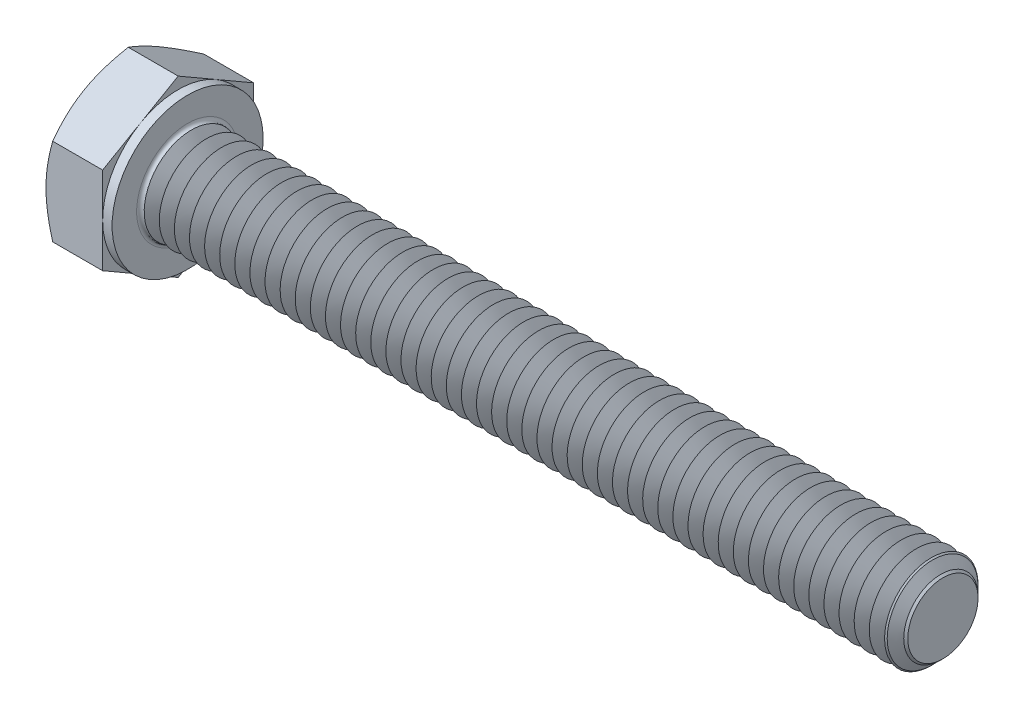
SolidWorks part; units mm, degrees
extrude "Boss-Extrude" add sketch "Sketch1" along normal blind 3.5
sketch "Sketch1" plane through (0, 0, 0) normal (1, 0, 0) x (0, 0, -1)
  line L0 (4, 2.3094) -> (4, -2.3094)
  line L1 (-4, 2.3094) -> (-4, -2.3094)
  line L2 (4, -2.3094) -> (0, -4.6188)
  line L3 (0, -4.6188) -> (-4, -2.3094)
  line L4 (4, 2.3094) -> (0, 4.6188)
  line L5 (0, 4.6188) -> (-4, 2.3094)
revolve "Cut-Revolve1" cut sketch "Sketch3" angle 360 about L6
sketch "Sketch3" plane through (0, 0, 0) normal (0, 0, 1) x (1, 0, 0)
  line L0 (0, 4) -> (3.244, 9.6188)
  line L1 (0, 4.6188) -> (0, 2.3094) construction
  line L2 (3.244, 9.6188) -> (3.244, 14.6188)
  line L3 (3.244, 14.6188) -> (-10, 14.6188)
  line L4 (-10, 14.6188) -> (-10, 4)
  line L5 (-10, 4) -> (0, 4)
  line L6 (0, 0) -> (99.06, 0) construction
  line L7 (3.5, 4.6188) -> (0, 4.6188) construction
revolve "Boss-Revolve1" add sketch "Sketch2" angle 360 about L7
sketch "Sketch2" plane through (0, 0, 0) normal (0, 0, 1) x (1, 0, 0)
  line L0 (0, 2.3094) -> (0, -2.3094) construction
  line L1 (0, 0) -> (43.5, 0)
  line L2 (0, 0) -> (0, 2.5)
  line L3 (0, 2.5) -> (43.5, 2.5)
  line L4 (43.5, 0) -> (43.5, 1.8072)
  line L5 (3.5, 4.6188) -> (3.5, 2.3094) construction
  line L7 (0, 0) -> (96.52, 0) construction
  line L8 (43.5, -1.8072) -> (90.335, -2.5) construction
  line L9 (0, -2.5) -> (90.335, -2.5) construction
  line L10 (4.3, 15.24) -> (4.3, -1.27) construction
  line L11 (3.5, 15.24) -> (3.5, -1.27) construction
  line L12 (3.5, 2.3094) -> (3.5, -2.3094) construction
  line L14 (43.5, 2.5) -> (43.5, 1.8072)
  dimension "l" = 40
  dimension "m" = 5
  dimension "Minor_dia" = 3.6144
  dimension "p" = 0.8
  dimension "h" = 40
cosmetic thread "Helix1" parameters "Thread_length"=39.2, "Thread_minor"=3.6144
ref_plane "Front Plane" through (0, 0, 0) normal (0, 0, 1) x (1, 0, 0)
ref_plane "Top Plane" through (0, 0, 0) normal (0, 1, 0) x (1, 0, 0)
ref_plane "Right Plane" through (0, 0, 0) normal (1, 0, 0) x (0, 0, -1)
sketch "Sketch5" plane through (0, 0, 0) normal (0, 0, 1) x (1, 0, 0)
  line L0 (3.5, 4) -> (0.256, 9.6188)
  line L1 (3.5, 4.6188) -> (3.5, 2.3094) construction
  line L2 (0.256, 9.6188) -> (0.256, 14.6188)
  line L3 (0.256, 14.6188) -> (10.256, 14.6188)
  line L4 (10.256, 14.6188) -> (10.256, 4)
  line L5 (10.256, 4) -> (3.5, 4)
  line L7 (3.5, 4.6188) -> (0.3573, 4.6188) construction
  line L8 (0, 0) -> (99.06, 0) construction
  line L9 (0, 0) -> (99.06, 0) construction
revolve "Cut-Revolve2" cut sketch "Sketch5" angle 360 about L8
sketch "Sketch4" plane through (0, 0, 0) normal (0, 0, 1) x (1, 0, 0)
  line L1 (3.5, 4.6188) -> (3.5, 2.3094) construction
  line L2 (3.5, 4) -> (3, 4)
  line L3 (3.5, 4) -> (3.5, 14.6188)
  line L4 (3.5, 14.6188) -> (3, 14.6188)
  line L5 (0, 0) -> (95.25, 0) construction
  line L6 (0, 0) -> (96.52, 0) construction
  line L7 (3, 4) -> (3, 14.6188)
  line L8 (3.1427, 4.6188) -> (0.3573, 4.6188) construction
revolve "Cut-Revolve3" cut sketch "Sketch4" angle 360 about L5
chamfer "Chamfer" distance 0.64 angle 45 1 edges at (43.5, 0, 2.5)
fillet "Fillet" radius 0.2 1 edges at (3.5, 0, -2.5)
sketch "Sketch6" plane through (0, 0, 0) normal (0, 0, 1) x (1, 0, 0)
  line L0 (4.1, -1.8072) -> (3.7, -2.5)
  line L1 (4.1, -1.8072) -> (4.5, -2.5)
  line L2 (4.5, -2.5) -> (4.5, -3.125)
  line L3 (-3.175, 0) -> (5.1513, 0) construction
  line L5 (4.5, -3.125) -> (3.7, -3.125)
  line L6 (3.7, -3.125) -> (3.7, -2.5)
  arc A0 (3.7, -2.5) -> (3.5, -2.7) centre (3.7, -2.7) ccw construction
revolve "Cut-Revolve4" cut sketch "Sketch6" angle 360 about L3
pattern_linear "LPattern1" count 50 spacing 0.8 along (1, 0, 0) of "Cut-Revolve4"
equation "\"D3@Sketch1\" = \"s@Sketch1\" / 2"
equation "\"D4@Sketch1\" = \"D3@Sketch1\""
equation "\"D5@Sketch1\" = \"D4@Sketch1\""
equation "\"D1@Sketch3\" = \"s@Sketch1\" / 2"
equation "\"D1@Sketch5\" = \"s@Sketch1\" / 2"
equation "\"Head_ch_ang@Sketch5\" = \"Head_ch_ang@Sketch3\""
equation "\"D1@Sketch4\" = \"s@Sketch1\""
equation "\"Diameter@Sketch6\" = \"m@Sketch2\""
equation "\"Overcut@Sketch6\" = \"m@Sketch2\" * 1.25"
equation "\"Minor_dia@Sketch2\" = \"m@Sketch2\"-\"p@Sketch2\" * 1.732"
equation "\"Thread_minor@Helix1\" = \"Minor_dia@Sketch2\""
equation "\"Thread_minor@Sketch6\" = \"Minor_dia@Sketch2\""
equation "\"D1@Chamfer\" = \"p@Sketch2\"*0.8"
equation "\"Thread_length@Helix1\" = \"l@Sketch2\" - \"p@Sketch2\""
equation "\"Num_threads@LPattern1\" = \"l@Sketch2\" / \"p@Sketch2\""
